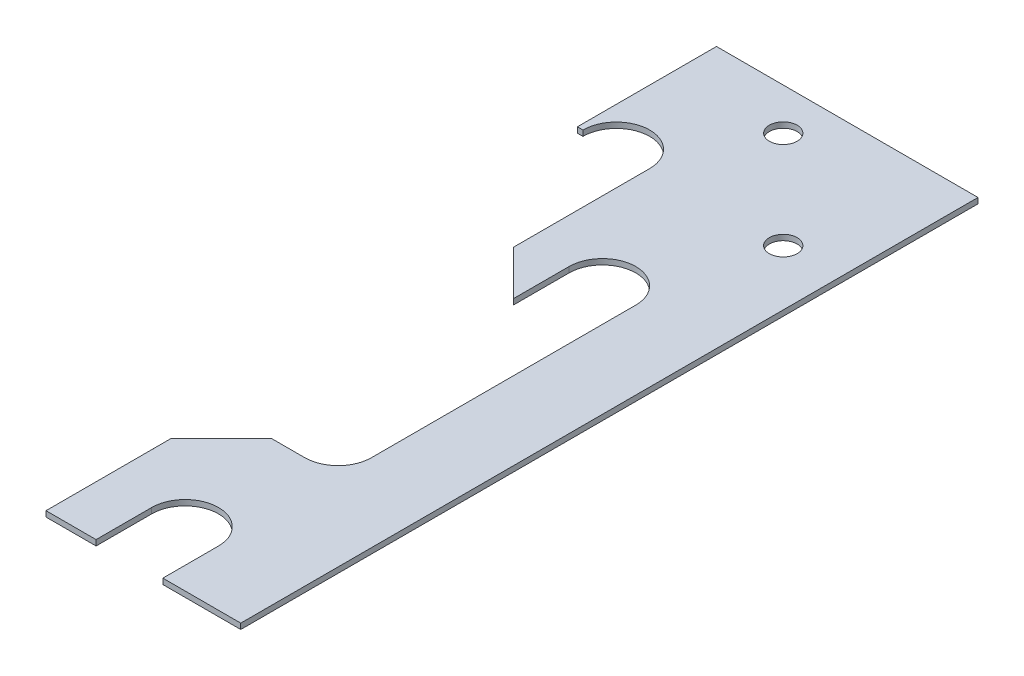
SolidWorks part; units mm, degrees
material "A3"
ref_plane "前视基准面" through (0, 0, 0) normal (0, 0, 1) x (1, 0, 0)
ref_plane "上视基准面" through (0, 0, 0) normal (0, 1, 0) x (1, 0, 0)
ref_plane "右视基准面" through (0, 0, 0) normal (1, 0, 0) x (0, 0, -1)
sketch "草图1" plane through (0, 0, 0) normal (0, 1, 0) x (1, 0, 0)
  line L0 (0, 0) -> (0, 50)
  line L1 (0, 50) -> (94, 50)
  line L2 (94, 50) -> (94, -215)
  line L3 (94, -215) -> (66, -215)
  line L4 (0, 0) -> (2, 0)
  line L5 (66, -45) -> (66, -140)
  line L6 (54, -152) -> (42, -152)
  line L7 (42, -152) -> (24, -170)
  line L8 (24, -170) -> (24, -215)
  line L9 (24, -215) -> (42, -215)
  line L10 (42, -215) -> (42, -195)
  line L11 (42, -195) -> (66, -195) construction
  line L12 (66, -195) -> (66, -215)
  line L13 (42, -45) -> (42, -65)
  line L14 (42, -65) -> (26, -49)
  line L15 (26, -49) -> (26, 0)
  arc A0 (26, 0) -> (2, 0) centre (14, 0) ccw
  arc A1 (66, -45) -> (42, -45) centre (54, -45) ccw
  circle A2 centre (39, 35) radius 5
  circle A3 centre (74, 0) radius 5
  arc A4 (66, -195) -> (42, -195) centre (54, -195) ccw
  arc A5 (66, -140) -> (54, -152) centre (54, -140) cw
  dimension "D4" = 12
  dimension "D5" = 12
  dimension "D6" = 10
  dimension "D7" = 24
  dimension "D18" = 150
  dimension "D20" = 12
  dimension "D22" = 45
  dimension "D1" = 94
  dimension "D2" = 265
  dimension "D3" = 50
  dimension "D8" = 70
  dimension "D9" = 45
  dimension "D10" = 63
  dimension "D11" = 45
  dimension "D12" = 40
  dimension "D13" = 40
  dimension "D14" = 20
  dimension "D15" = 50
  dimension "D16" = 55
  dimension "D17" = 15
  dimension "D19" = 24
  dimension "D21" = 20
extrude "凸台-拉伸1" add sketch "草图1" along normal blind 2
